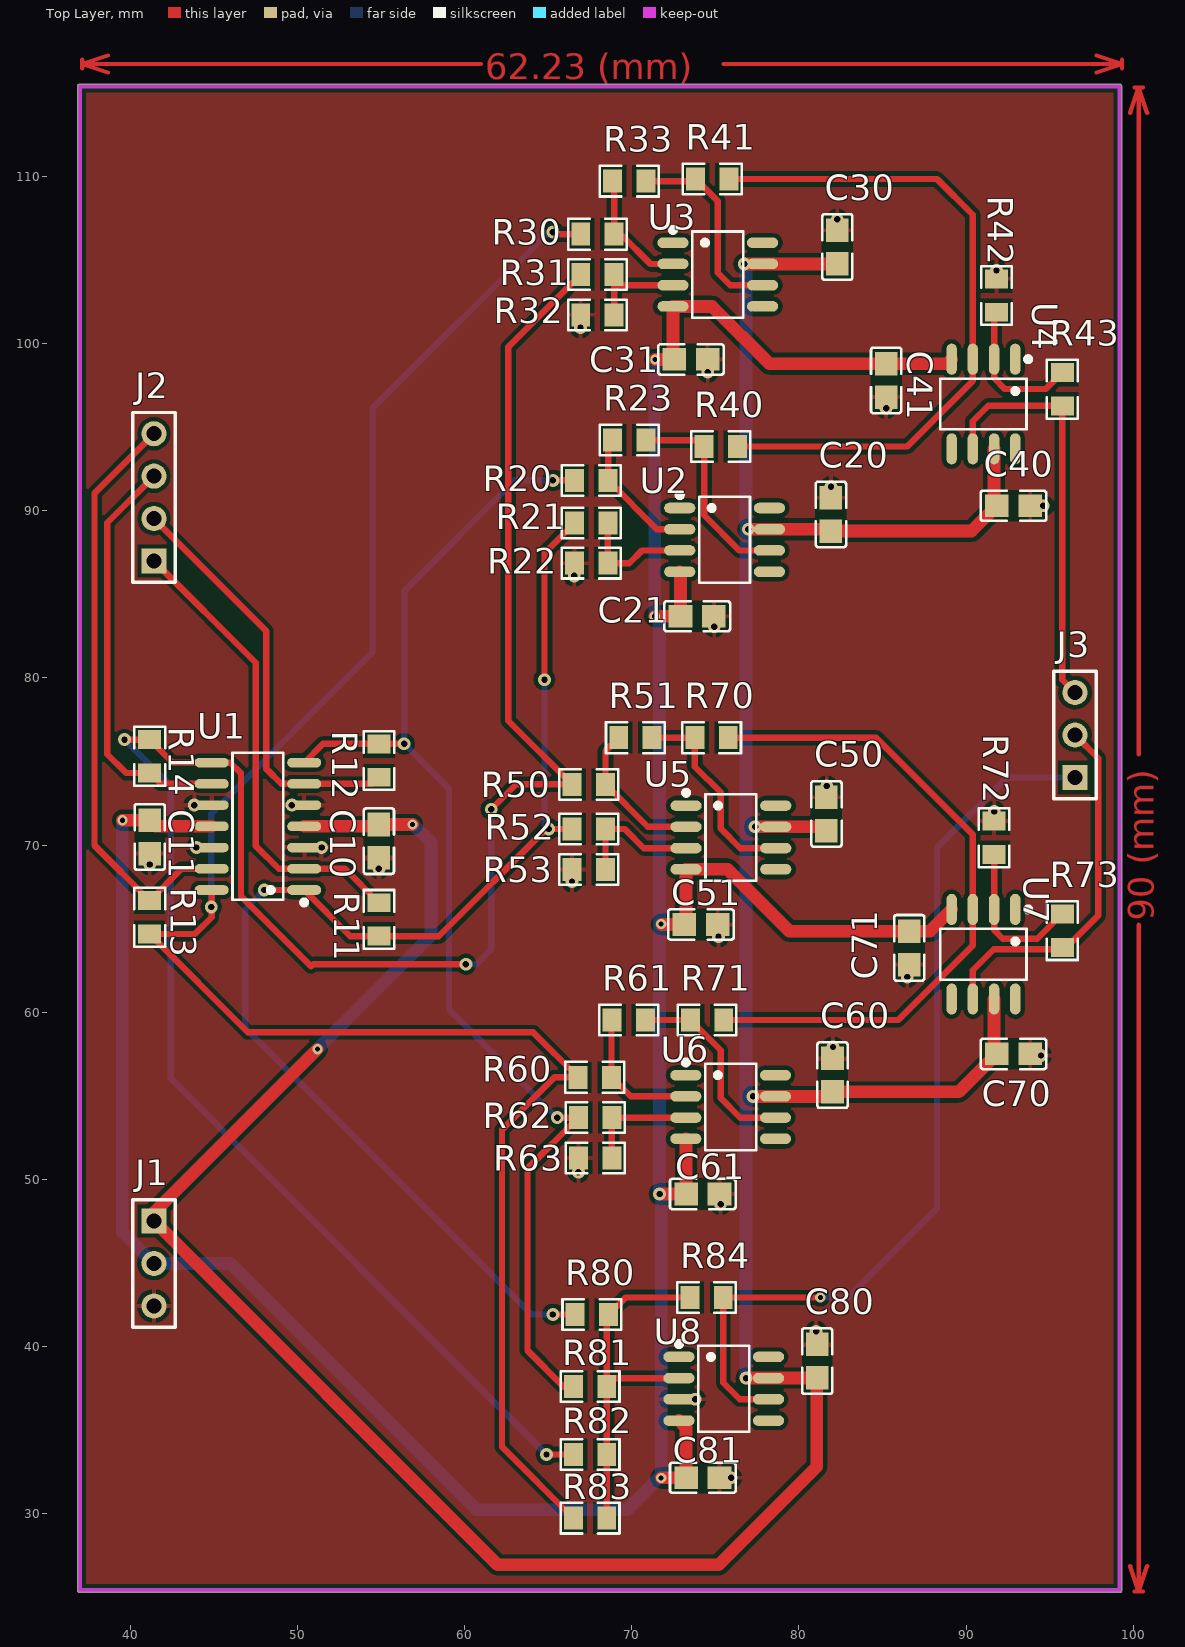
[diagram p0: Top Layer view]
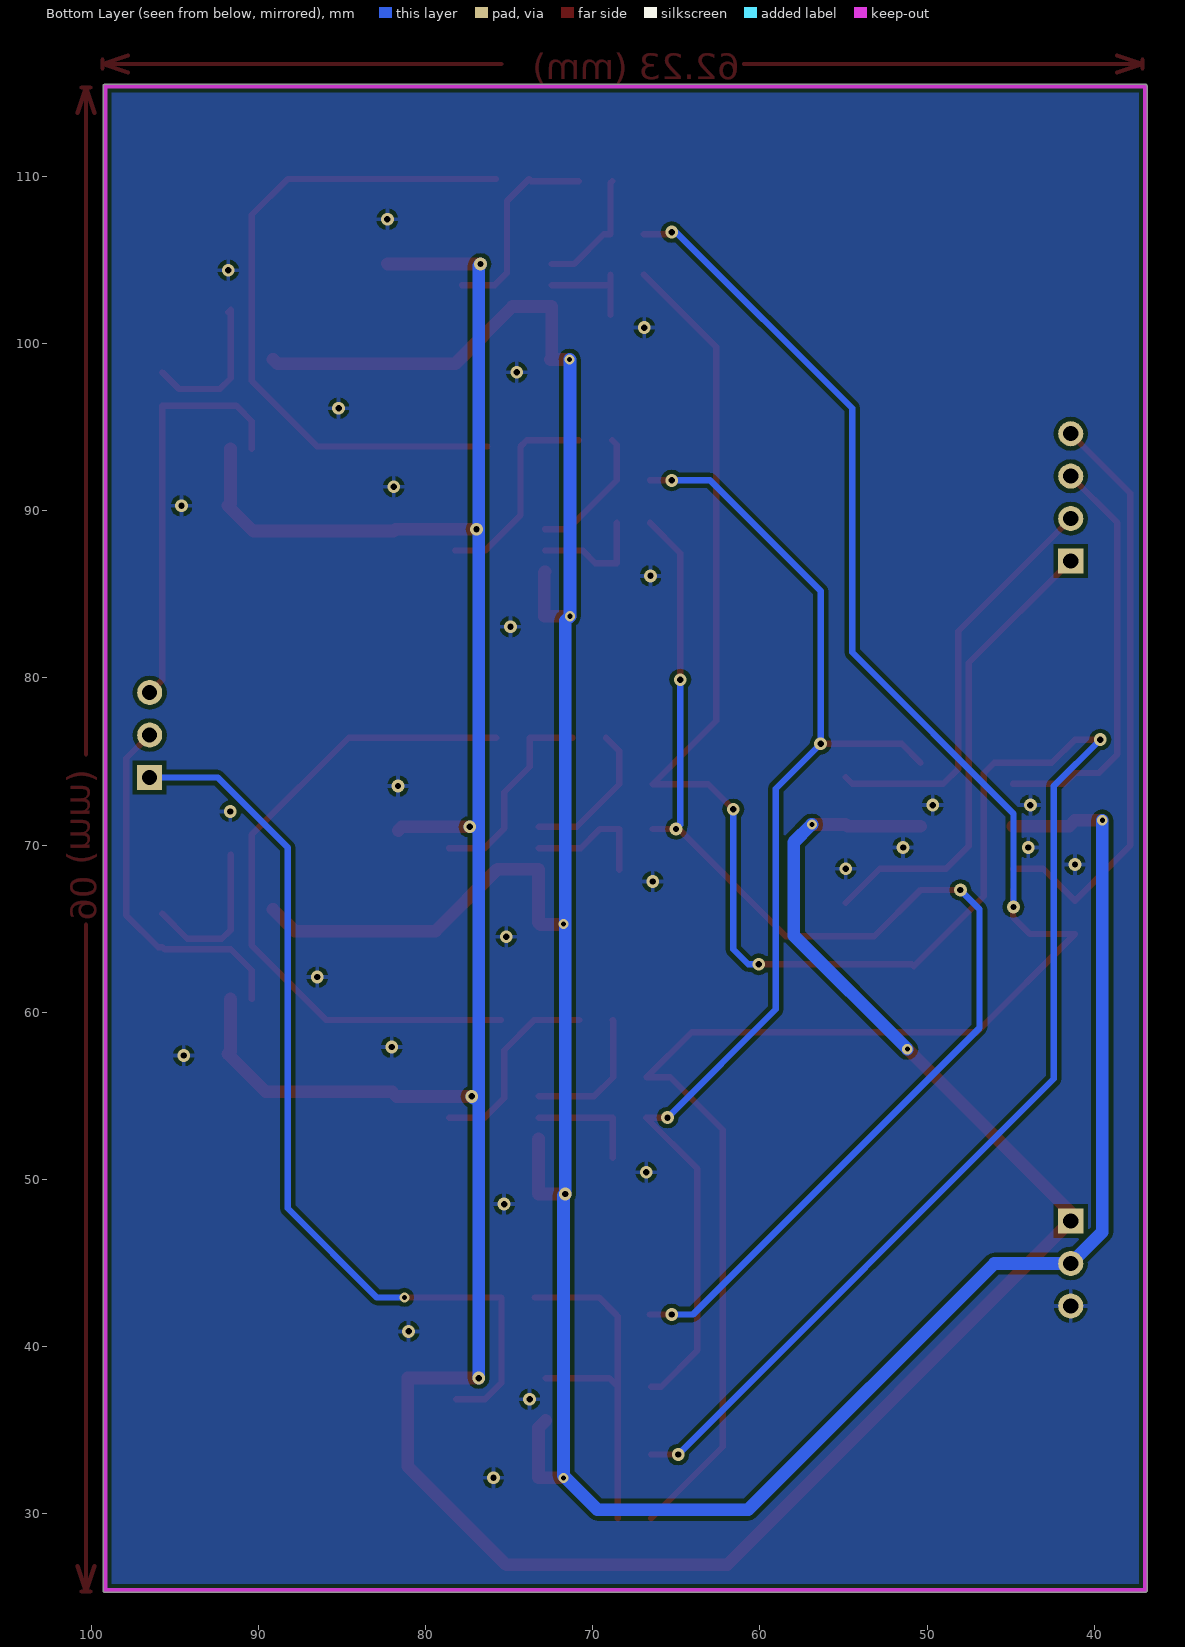
[diagram p1: Bottom Layer view, seen from below]
# Altium PCB MISC68795.PcbDoc
Units mm, origin at the board's own origin, x right, y up, seen from the top; angles counter-clockwise.
Board outline 62.48 x 90.25 mm, 2 copper layers (Top Layer, Bottom Layer); 60 components, 31 nets, 178 pads, 54 vias.

## Layer stack, top to bottom (the 12.6 mil dielectric is the usual default, probably not edited)
Top Solder: solder mask 0.0102, Solder Resist, Dk 3.5
Top Layer: signal copper 0.0356
Dielectric 1: dielectric 0.32, FR-4, Dk 4.8
Bottom Layer: signal copper 0.0356
Bottom Solder: solder mask 0.0102, Solder Resist, Dk 3.5

## Board outline
36.83,25.4 ccw(c36.957,25.4) 36.957,25.273 99.187,25.273 ccw(c99.187,25.4) 99.314,25.4 99.314,115.4 ccw(c99.187,115.4) 99.187,115.527 36.957,115.527 ccw(c36.957,115.4) 36.83,115.4

## Design rules (kind name [scope] priority, off if disabled: settings)
Clearance [All] p1: gap=0.254
MinimumSolderMaskSliver [All] p1: minsoldermaskwidth=0
PolygonConnect [All] p1: connectstyle=Relief reliefconductorwidth=0.254 reliefentries=4 polygonreliefangle="90 Angle" airgapwidth=0.254
RoutingVias [All] p1: holewidth=0.711 width=1.27 viastyle="Through Hole" minholewidth=0.711 minwidth=1.27 maxholewidth=0.711 maxwidth=1.27
SilkToSilkClearance [All] p1: silktosilkclearance=0
SilkToSolderMaskClearance [IsPad] p1: minsilkscreentomaskgap=0 clearancetoexposedcopper=TRUE
SolderMaskExpansion [All] p1: expansion=0.102
Width [All] p1: maxlimit=0.762 minlimit=0.254 preferedwidth=0.254
27 further rules are at their usual default settings.

## Components (designator, comment, footprint, x,y, rotation, side; value= is the part's Value field where it differs from the comment)
C10 "0.1uF" C0805 54.864,70.231 r90 top
C11 "0.1uF" C0805 41.148,70.485 r90 top
C20 "0.1uF" C0805 81.915,89.789 r90 top
C21 "0.1uF" C0805 73.914,83.693 r0 top
C30 "0.1uF" C0805 82.296,105.791 r90 top
C31 "0.1uF" C0805 73.533,99.06 r0 top
C40 "0.1uF" C0805 92.837,90.297 r0 top
C41 "0.1uF" C0805 85.217,97.806 r270 top
C50 "0.1uF" C0805 81.645,71.866 r90 top
C51 "0.1uF" C0805 74.136,65.246 r0 top
C60 "0.1uF" C0805 82.01,56.229 r90 top
C61 "0.1uF" C0805 74.247,49.117 r0 top
C70 "0.1uF" C0805 92.837,57.499 r0 top
C71 "0.1uF" C0805 86.598,63.849 r270 top
C80 "0.1uF" C0805 81.089,39.116 r90 top
C81 "0.1uF" C0805 74.247,32.131 r0 top
J1 "电源" HDR1X3 41.402,47.498 r270 top
J2 "四路信号输入" HDR1X4 41.402,86.995 r90 top
J3 "输出" HDR1X3 96.52,74.041 r90 top
R11 "3K" R0805 54.864,65.548 r270 top
R12 "3K" R0805 54.864,75.057 r90 top
R13 "3K" R0805 41.148,65.675 r90 top
R14 "3K" R0805 41.148,75.311 r270 top
R20 "10K" R0805 67.58,91.821 r0 top
R21 "10K" R0805 67.58,89.281 r0 top
R22 "10K" R0805 67.564,86.868 r0 top
R23 "10K" R0805 69.85,94.234 r0 top
R30 "10K" R0805 67.945,106.553 r0 top
R31 "10K" R0805 67.945,104.14 r0 top
R32 "10K" R0805 67.945,101.727 r0 top
R33 "10K" R0805 69.85,109.728 r0 top
R40 "10K" R0805 75.327,93.853 r0 top
R41 "10K" R0805 74.819,109.855 r0 top
R42 "10K" R0805 91.821,102.886 r270 top
R43 "10K" R0805 95.758,97.282 r90 top
R50 "10K" R0805 67.421,73.628 r0 top
R51 "10K" R0805 70.215,76.422 r0 top
R52 "10K" R0805 67.421,70.961 r0 top
R53 "10K" R0805 67.421,68.53 r0 top
R60 "10K" R0805 67.786,56.102 r0 top
R61 "10K" R0805 69.818,59.531 r0 top
R62 "10K" R0805 67.802,53.689 r0 top
R63 "10K" R0805 67.802,51.276 r0 top
R70 "10K" R0805 74.771,76.422 r0 top
R71 "10K" R0805 74.501,59.531 r0 top
R72 "10K" R0805 91.678,70.437 r270 top
R73 "10K" R0805 95.758,64.881 r90 top
R80 "10k" R0805 67.611,41.91 r0 top
R81 "10k" R0805 67.5,37.592 r0 top
R82 "10k" R0805 67.5,33.528 r0 top
R83 "10k" R0805 67.5,29.718 r0 top
R84 "10k" R0805 74.469,42.926 r0 top
U1 "OPA4131" SOIC-14_L8.7-W3.9-P1.27-LS6.0-BL 47.625,71.12 r90 top
U2 "OP07" SOP-8_L4.9-W3.9-P1.27-LS6.0-BL 75.55,88.265 r270 top
U3 "OP07" SOP-8_L4.9-W3.9-P1.27-LS6.0-BL 75.145,104.14 r270 top
U4 "OP07" SOP-8_L4.9-W3.9-P1.27-LS6.0-BL 91.043,96.393 r180 top
U5 "OP07" SOP-8_L4.9-W3.9-P1.27-LS6.0-BL 75.93,70.453 r270 top
U6 "OP07" SOP-8_L4.9-W3.9-P1.27-LS6.0-BL 75.914,54.324 r270 top
U7 "OP07" SOP-8_L4.9-W3.9-P1.27-LS6.0-BL 91.043,63.468 r180 top
U8 "OP07" SOP-8_L4.9-W3.9-P1.27-LS6.0-BL 75.501,37.465 r270 top

## Footprints (in the part's own frame and the unit in brackets; to place one, negate y for a bottom-side part, rotate by r counter-clockwise, add the part's x,y. Pads: shape width x height; smd on the part's side, far side on the other; paste and mask are expansions set on the pad)
C0805 [mm]
  rect 1.41x1.35 smd paste-100 mask+0.051: 1(-1,0) 2(1,0)
  silkscreen extent -1.96,-0.9 1.96,0.9
HDR1X3 [mm] "Connector; Header; 3 Position"
  rect 1.5x1.5 hole 0.9: 1(0,0)
  round 1.5 hole 0.9: 2(2.54,0) 3(5.08,0)
  silkscreen extent -1.27,-1.27 6.35,1.27
HDR1X4 [mm] "Connector; Header; 4 Position"
  rect 1.5x1.5 hole 0.9: 1(0,0)
  round 1.5 hole 0.9: 2(2.54,0) 3(5.08,0) 4(7.62,0)
  silkscreen extent -1.27,-1.27 8.89,1.27
R0805 [mm]
  rect 1.133x1.377 smd paste-100 mask+0.051: 1(-1,0) 2(1,0)
  silkscreen extent -1.76,-0.92 1.76,0.92
SOIC-14_L8.7-W3.9-P1.27-LS6.0-BL [mm]
  oval 0.574x2.038 smd: 1(-3.81,-2.769) 2(-2.54,-2.769) 3(-1.27,-2.769) 4(0,-2.769) 5(1.27,-2.769) 6(2.54,-2.769) 7(3.81,-2.769) 8(3.81,2.769) 9(2.54,2.769) 10(1.27,2.769) 11(0,2.769) 12(-1.27,2.769) 13(-2.54,2.769) 14(-3.81,2.769)
  silkscreen extent -4.7,-2.92 4.4,1.52
SOP-8_L4.9-W3.9-P1.27-LS6.0-BL [mm]
  oval 0.63x1.865 smd: 1(-1.905,-2.682) 2(-0.635,-2.682) 3(0.635,-2.682) 4(1.905,-2.682) 5(1.905,2.682) 6(0.635,2.682) 7(-0.635,2.682) 8(-1.905,2.682)
  silkscreen extent -2.82,-2.83 2.58,1.52

## Part data
C10 C11 C20 C21 C30 C31 C40 C41 C50 C51 C60 C61 C70 C71 C80 C81: library part Cap, "Capacitor"
J2: library part CON4
J3: library part 电源
R11 R12 R13 R14 R20 R21 R22 R23 R30 R31 R32 R33 R40 R41 R42 R43 R50 R51 R52 R53 R60 R61 R62 R63 R70 R71 R72 R73 R80 R81 R82 R83 R84: library part Res2, "Resistor"

## Via types
v1: diameter 0.762, hole 0.381, Top Layer to Bottom Layer, 46 vias
v2: diameter 0.61, hole 0.305, Top Layer to Bottom Layer, 8 vias

## Nets (pads, with @x,y where several pads share a name; then routed paths per layer and width w, separated by ;. In a path a pad name is that pad's centre, name@x,y a point inside that pad or via, vN(x,y) a via of type N, cw(c..) or ccw(c..) an arc to the next point about the centre after c; other vN are vias at no path point)
+15V: C10.2 C20.1 C30.1 C40.1 C50.1 C60.1 C70.1 C80.1 J1.1 U1.4 U2.7 U3.7 U4.7 U5.7 U6.7 U7.7 U8.7 | length 213.5
  Top Layer w0.762: U1.4 54.753,71.12 C10.2 v2(56.88,71.231) ; v2(51.181,57.785) 41.402,48.006 J1.1 61.976,26.924 75.184,26.924 81.073,32.813 81.073,38.1 U8.7 v1(76.835,38.1) ; v1(76.724,104.775) U3.7 82.28,104.775 C30.1 ; v1(76.962,88.9) U2.7 81.804,88.9 C20.1 90.329,88.789 C40.1 91.678,90.456 U4.7 ; v1(77.248,54.959) U6.7 81.74,54.959 C60.1 89.567,55.229 C70.1 91.678,57.658 U7.7 ; v1(77.375,71.088) U5.7 81.423,71.088 C50.1
  Bottom Layer w0.762: v2(51.181,57.785) 57.975,64.579 57.975,70.168 56.912,71.231 v2(56.88,71.231) ; v1(76.724,104.775) 76.835,104.664 76.835,71.247 ; v1(76.835,38.1) 76.835,54.864 ; v1(77.248,54.959) 77.153,54.864 76.835,54.864 ; v1(77.375,71.088) 76.994,71.088 76.835,71.247 ; 76.835,54.864 76.835,71.247
-15V: C11.2 C21.1 C31.1 C41.1 C51.1 C61.1 C71.1 C81.1 J1.2 U1.11 U2.4 U3.4 U4.4 U5.4 U6.4 U7.4 U8.4 | length 196.5
  Top Layer w0.762: v2(39.513,71.485) C11.2 41.513,71.12 U1.11 ; v2(71.374,83.693) C21.1 72.914,86.313 U2.4 ; v2(71.389,99.06) C31.1 72.462,99.131 U3.4 74.803,102.235 78.232,98.806 C41.1 88.869,98.806 U4.4 ; v1(71.66,49.117) C61.1 73.247,52.404 U6.4 ; v2(71.755,32.131) C81.1 73.247,35.132 U8.4 ; v2@71.787,65.246 C51.1 73.248,65.358 U5.4 75.724,68.548 79.423,64.849 C71.1 87.837,64.849 U7.4
  Bottom Layer w0.762: v2(39.513,71.485) 39.513,46.847 J1.2 45.974,44.958 60.706,30.226 69.723,30.226 71.755,32.258 71.755,49.022 v1(71.66,49.117) 71.66,83.407 v2(71.374,83.693) 71.374,99.045 v2(71.389,99.06)
  other v2: 71.755,65.278
GND: C10.1 C11.1 C20.2 C21.2 C30.2 C31.2 C40.2 C41.2 C50.2 C51.2 C60.2 C61.2 C70.2 C71.2 C80.2 C81.2 J1.3 R22.1 R32.1 R42.1 R53.1 R63.1 R72.1 U1.3 U1.5 U1.10 U1.12 U8.3
  other v1: 75.946,32.131 73.787,36.83 81.026,40.894 75.311,48.514 66.802,50.419 94.488,57.404 82.042,57.912 86.487,62.103 75.184,64.516 66.421,67.818 54.864,68.58 41.148,68.834 43.942,69.85 51.435,69.85 91.694,72.009 43.815,72.39 49.657,72.39 81.661,73.533 74.93,83.058 66.548,86.106 94.615,90.297 81.915,91.44 85.217,96.139 74.549,98.298 66.929,100.965 91.821,104.394 82.296,107.442
InA: J2.1 R11.1 U1.2 | length 28.3
  Top Layer w0.381: J2.1 47.498,80.899 47.498,69.945 48.863,68.58 U1.2 52.832,68.58 R11.1
InB: J2.2 R12.1 U1.6 | length 25
  Top Layer w0.381: J2.2 48.133,82.804 48.133,74.549 49.022,73.66 U1.6 54.467,73.66 R12.1
InC: J2.3 R14.2 U1.9 | length 24.8
  Top Layer w0.381: J2.3 38.608,89.281 38.608,75.438 39.735,74.311 R14.2 41.799,73.66 U1.9
InD: J2.4 R13.2 U1.13 | length 35.3
  Top Layer w0.381: J2.4 37.846,91.059 37.846,69.977 R13.2 43.053,68.58 U1.13
NetR20_2: R20.2 R23.1 U2.2 | length 8
  Top Layer w0.381: R23.1 68.58,93.964 R20.2 71.501,88.9 U2.2
NetR21_2: R21.2 R22.2 U2.3 | length 7
  Top Layer w0.381: R21.2 68.564,89.265 R22.2 69.85,86.868 70.612,87.63 U2.3
NetR23_2: R23.2 R40.1 U2.6 | length 12.5
  Top Layer w0.381: R23.2 73.946,94.234 R40.1 74.327,89.741 76.438,87.63 U2.6
NetR30_2: R30.2 R33.1 U3.2 | length 7.5
  Top Layer w0.381: R33.1 68.945,109.633 R30.2 69.342,106.553 71.12,104.775 U3.2
NetR31_2: R31.2 R32.2 U3.3 | length 5.9
  Top Layer w0.381: R32.2 R31.2@68.945,103.505 ; R31.2 R31.2@68.945,103.505 ; U3.3 R31.2@68.945,103.505
NetR33_2: R33.2 R41.1 U3.6 | length 12.2
  Top Layer w0.381: R33.2 73.692,109.728 R41.1 75.136,108.538 75.136,104.251 75.882,103.505 U3.6
NetR40_2: R40.2 R41.2 U4.3 | length 41.1
  Top Layer w0.381: R41.2 88.265,109.855 90.408,107.712 U4.3 90.408,97.774 86.487,93.853 R40.2
NetR42_2: R42.2 R43.2 U4.2 | length 9.1
  Top Layer w0.381: R42.2 91.678,102.029 U4.2 91.678,97.933 92.318,97.293 94.769,97.293 R43.2
NetR50_2: R50.2 R51.1 U5.2 | length 9
  Top Layer w0.381: R51.1 68.421,75.628 R50.2 70.961,71.088 U5.2
NetR51_2: R51.2 R70.1 U5.6 | length 12.4
  Top Layer w0.381: R51.2 R70.1 73.771,74.692 75.311,73.152 75.311,70.993 76.486,69.818 U5.6
NetR52_2: R52.2 R53.2 U5.3 | length 7.7
  Top Layer w0.381: R53.2 R52.2 69.58,70.961 70.723,69.818 U5.3
NetR60_2: R60.2 R61.1 U6.2 | length 8.4
  Top Layer w0.381: R61.1 68.786,59.499 R60.2 69.929,54.959 U6.2
NetR61_2: R61.2 R71.1 U6.6 | length 11.9
  Top Layer w0.381: R61.2 R71.1 75.311,57.721 75.311,54.864 76.486,53.689 U6.6
NetR62_2: R62.2 R63.2 U6.3 | length 6.8
  Top Layer w0.381: R63.2 R62.2 U6.3
NetR70_2: R70.2 R71.2 U7.3 | length 40.4
  Top Layer w0.381: R71.2 85.947,59.531 90.408,63.992 U7.3 90.408,70.628 84.614,76.422 R70.2
NetR72_2: R72.2 R73.2 U7.2 | length 9.4
  Top Layer w0.381: R72.2 U7.2 91.678,64.913 92.202,64.389 94.266,64.389 R73.2
NetR80_2: R80.2 R81.2 R82.2 R83.2 R84.1 U8.2 | length 22
  Top Layer w0.381: R83.2 R82.2 R81.2 ; U8.2 69.008,38.1 R81.2 ; R84.1 69.627,42.926 R80.2 68.5,41.799 R81.2
OUT: J3.1 R84.2 U8.6 | length 54.8
  Top Layer w0.381: U8.6 76.454,36.83 75.469,37.815 R84.2 v2(81.28,42.926)
  Bottom Layer w0.381: v2(81.28,42.926) 82.931,42.926 88.265,48.26 88.265,69.85 92.456,74.041 J3.1
OutA: R11.2 R21.1 R52.1 R80.1 U1.1 | length 77
  Top Layer w0.381: v1(48.006,67.31) U1.1 53.156,64.548 R11.2 58.452,64.548 64.865,70.961 v1(65.024,70.961) R52.1 ; v1(64.77,79.899) 64.77,87.471 R21.1 ; v1(65.278,41.91) R80.1
  Bottom Layer w0.381: v1(48.006,67.31) 46.863,66.167 46.863,59.055 64.008,41.91 v1(65.278,41.91) ; v1(64.77,79.899) 64.77,71.215 v1(65.024,70.961)
OutB: R12.2 R20.1 R62.1 R81.1 U1.7 | length 74.8
  Top Layer w0.381: U1.7 51.521,76.057 R12.2 v1(56.372,76.057) ; v1(65.278,91.821) R20.1 ; v1(65.532,53.689) R62.1 63.754,50.641 63.754,39.751 65.913,37.592 R81.1
  Bottom Layer w0.381: v1(65.278,91.821) 62.992,91.821 56.372,85.201 v1(56.372,76.057) 59.055,73.374 59.055,60.166 v1(65.532,53.689)
OutC: R14.1 R31.1 R50.1 R82.1 U1.8 | length 134.9
  Top Layer w0.381: v1(39.64,76.311) R14.1 42.529,74.93 U1.8 45.974,74.93 46.609,74.295 46.609,66.929 50.8,62.738 50.927,62.865 v1(60.071,62.865) ; v1(61.595,72.136) 63.087,73.628 R50.1 62.611,77.438 62.611,99.806 R31.1 ; v1(64.897,33.528) R82.1
  Bottom Layer w0.381: v1(39.64,76.311) 42.418,73.533 42.418,56.007 v1(64.897,33.528) ; v1(60.071,62.865) 60.706,62.865 61.595,63.754 v1(61.595,72.136)
OutD: R13.1 R30.1 R60.1 R83.1 U1.14 | length 116.5
  Top Layer w0.381: U1.14 44.856,65.684 43.847,64.675 R13.1 47.022,58.801 64.087,58.801 R60.1 65.373,56.102 62.23,52.959 62.23,33.988 R83.1 ; v1(65.278,106.68) 65.405,106.553 R30.1
  Bottom Layer w0.381: v1(44.831,66.294) 44.831,71.882 54.483,81.534 54.483,96.139 65.024,106.68 v1(65.278,106.68)
Ux: J3.3 R43.1 U4.6 | length 24.9
  Top Layer w0.381: U4.6 90.408,95.361 91.329,96.282 R43.1 95.758,79.883 J3.3
Uy: J3.2 R73.1 U7.6 | length 22
  Top Layer w0.381: U7.6 90.408,62.5 91.662,63.754 95.631,63.754 R73.1 96.012,63.881 97.917,65.786 97.917,75.184 J3.2
pads on no net: U2.1 U2.5 U2.8 U3.1 U3.5 U3.8 U4.1 U4.5 U4.8 U5.1 U5.5 U5.8 U6.1 U6.5 U6.8 U7.1 U7.5 U7.8 U8.1 U8.5 U8.8
copper on no net: | length 142.4
  Top Layer w0.254: 37.107,116.484 37.107,116.992 ; 38.631,116.23 37.107,116.738 ; 38.631,117.246 37.107,116.738 ; 60.96,116.738 37.107,116.738 ; 75.484,116.738 99.337,116.738 ; 97.813,116.23 99.337,116.738 ; 97.813,117.246 99.337,116.738 ; 99.337,116.484 99.337,116.992 ; 99.822,26.858 100.33,25.334 ; 99.822,113.81 100.33,115.334 ; 100.076,25.334 100.584,25.334 ; 100.076,115.334 100.584,115.334 ; 100.33,65.23 100.33,25.334 ; 100.33,75.438 100.33,115.334 ; 100.838,26.858 100.33,25.334 ; 100.838,113.81 100.33,115.334

## Polygon pours and split planes (outlines as drawn)
GND on Bottom Layer "G" (solid, remove dead copper, pour order 6): 17.145,116.586 26.416,125.857 107.823,125.857 107.823,13.462 107.569,13.208 105.791,11.43 23.495,11.43
GND on Top Layer "G" (solid, remove dead copper, pour order 12): 28.575,124.841 110.617,124.841 111.252,125.476 113.157,123.571 113.157,7.366 33.147,7.366 22.352,18.161

## Keep-outs
Keep-Out Layer:
  lines w0.254: 36.957,25.4 36.957,71.247 36.957,115.4 99.187,115.4 99.187,73.025 99.187,25.4 36.957,25.4

## Other copper
Top Layer:
  text "62.23 (mm)" at 61.214,115.824 h1.52
  text "90 (mm)" at 101.244,65.484 h1.52 r90